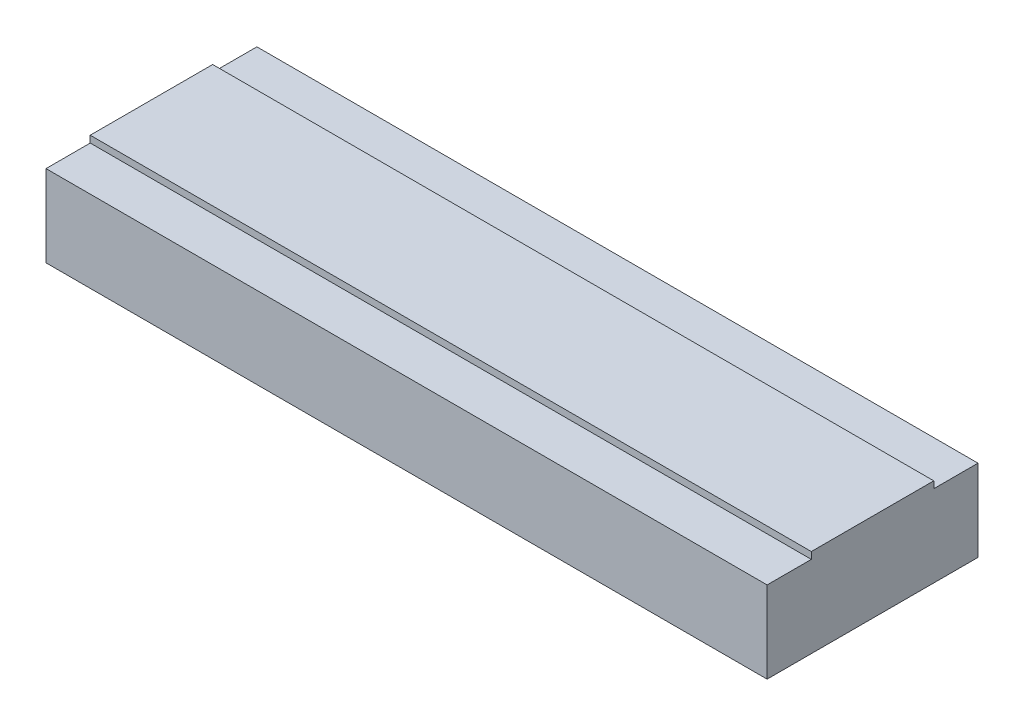
from build123d import *

# Parameters (mm, degrees)
SKETCH1_W           = 212
SKETCH1_H           = 62
BOSS_EXTRUDE1_DEPTH = 26
SHELL1_T            = -7.5
SKETCH2_W           = 13
SKETCH2_H           = 2
CUT_EXTRUDE2_DEPTH  = 216.826319062
RIB1_REACH          = 115.459
SKETCH3_WALLS_W     = 6
SKETCH3_WALLS_H     = 275.918487568
SKETCH3_WALLS_H_2   = 275.934517232
BOSS_EXTRUDE2_REACH = 115.459


with BuildPart() as part:
    # Sketch1 → Boss-Extrude1 (new body)
    with BuildSketch(Plane(origin=(0, 0, 0), x_dir=(1, 0, 0), z_dir=(0, 1, 0))):
        Rectangle(SKETCH1_W, SKETCH1_H)
    extrude(amount=BOSS_EXTRUDE1_DEPTH)

    # Shell1
    shell1_openings = [part.faces().sort_by_distance(p)[0] for p in [
        (0, 0, 0),
    ]]
    offset(amount=SHELL1_T, openings=shell1_openings, kind=Kind.INTERSECTION)

    # Sketch2 → Cut-Extrude2 (cut, through all)
    with BuildSketch(Plane(origin=(106, 0, 0), x_dir=(0, 0, -1), z_dir=(1, 0, 0))):
        with Locations((24.5, 25)):
            Rectangle(SKETCH2_W, SKETCH2_H)
        with Locations((-24.5, 25)):
            Rectangle(SKETCH2_W, SKETCH2_H)
    extrude(amount=-CUT_EXTRUDE2_DEPTH, mode=Mode.SUBTRACT)

    # Sketch3 walls → Rib1 (add, up to next)
    with BuildSketch(Plane.XZ, mode=Mode.PRIVATE) as rib1_sk1:
        with Locations((45.5, 0)):
            Rectangle(SKETCH3_WALLS_W, SKETCH3_WALLS_H)
    rib1_tool1 = extrude(rib1_sk1.sketch, amount=-RIB1_REACH, mode=Mode.PRIVATE) - part.part
    # Sketch3 walls → Rib1 (add, up to next)
    with BuildSketch(Plane.XZ, mode=Mode.PRIVATE) as rib1_sk2:
        with Locations((-45.5, 0.008014832)):
            Rectangle(SKETCH3_WALLS_W, SKETCH3_WALLS_H_2)
    rib1_tool2 = extrude(rib1_sk2.sketch, amount=-RIB1_REACH, mode=Mode.PRIVATE) - part.part
    add(rib1_tool1.solids().sort_by_distance((45.5, 0, 0))[0])
    add(rib1_tool2.solids().sort_by_distance((-45.5, 0, 0.008014832))[0])

    # Sketch4 → Boss-Extrude2 (add, up to next)
    with BuildSketch(Plane.XZ, mode=Mode.PRIVATE) as boss_extrude2_sk1:
        Polygon((86.5, 23.5), (98.5, 11.5), (98.5, 23.5), align=None)
    boss_extrude2_tool1 = extrude(boss_extrude2_sk1.sketch, amount=-BOSS_EXTRUDE2_REACH, mode=Mode.PRIVATE) - part.part
    # Sketch4 → Boss-Extrude2 (add, up to next)
    with BuildSketch(Plane.XZ, mode=Mode.PRIVATE) as boss_extrude2_sk2:
        Polygon((-98.5, -11.5), (-86.5, -23.5), (-98.5, -23.5), align=None)
    boss_extrude2_tool2 = extrude(boss_extrude2_sk2.sketch, amount=-BOSS_EXTRUDE2_REACH, mode=Mode.PRIVATE) - part.part
    add(boss_extrude2_tool1.solids().sort_by_distance((94.5, 0, 19.5))[0])
    add(boss_extrude2_tool2.solids().sort_by_distance((-94.5, 0, -19.5))[0])


solid = part.part
